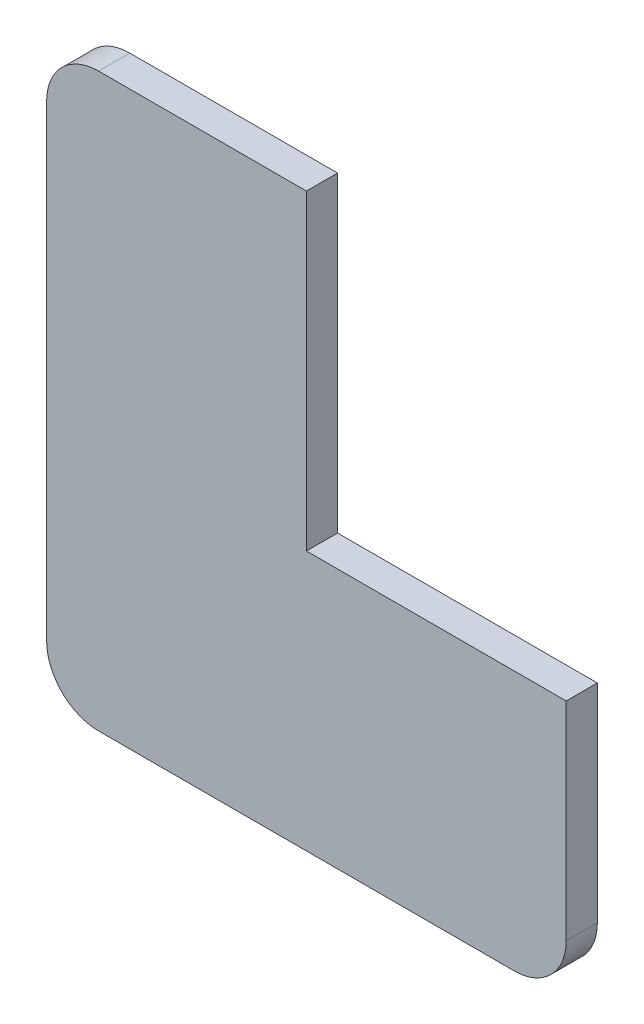
from build123d import *

# Parameters (mm, degrees)
BOSS_EXTRUDE1_DEPTH = 3


with BuildPart() as part:
    # Sketch1 → Boss-Extrude1 (new body)
    with BuildSketch(Plane.XY):
        with BuildLine():
            Line((-360, -3), (-385, -3))
            Line((-385, -3), (-385, 27))
            Line((-385, 27), (-405, 27))
            ThreePointArc((-405, 27), (-408.535533906, 25.535533906), (-410, 22))
            Line((-410, 22), (-410, -3))
            Line((-410, -3), (-410, -23))
            ThreePointArc((-410, -23), (-408.535533906, -26.535533906), (-405, -28))
            Line((-405, -28), (-365, -28))
            ThreePointArc((-365, -28), (-361.464466094, -26.535533906), (-360, -23))
            Line((-360, -23), (-360, -3))
        make_face()
    extrude(amount=BOSS_EXTRUDE1_DEPTH)


solid = part.part
